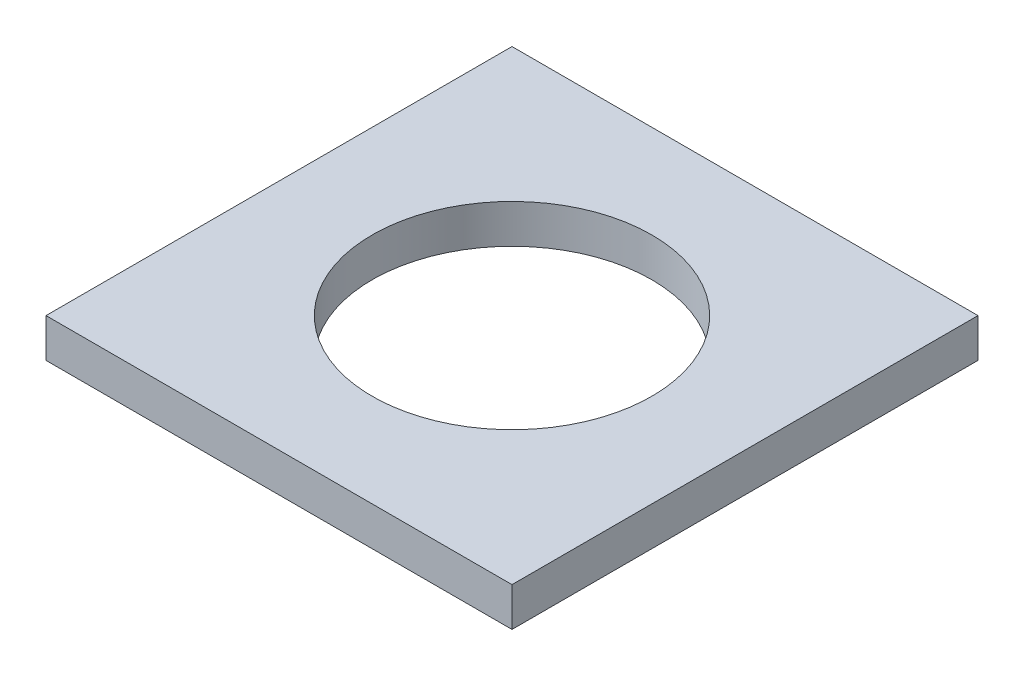
SolidWorks part; units mm, degrees
ref_plane "Front Plane" through (0, 0, 0) normal (0, 0, 1) x (1, 0, 0)
ref_plane "Top Plane" through (0, 0, 0) normal (0, 1, 0) x (1, 0, 0)
ref_plane "Right Plane" through (0, 0, 0) normal (1, 0, 0) x (0, 0, -1)
ref_plane "Plane1" through (0, 819.8956, 0) normal (0, 1, 0) x (1, 0, 0)
sketch "Sketch1" plane through (0, 819.8956, 0) normal (0, 1, 0) x (1, 0, 0)
  line L0 (581.2306, 380.693) -> (581.2306, 500.693)
  line L1 (581.2306, 500.693) -> (461.2306, 500.693)
  line L2 (461.2306, 500.693) -> (461.2306, 380.693)
  line L3 (461.2306, 380.693) -> (581.2306, 380.693)
  circle A0 centre (521.2306, 440.693) radius 36
  dimension "D1" = 72
  dimension "D2" = 60
  dimension "D3" = 120
  dimension "D4" = 60
  dimension "D5" = 120
extrude "Boss-Extrude1" add sketch "Sketch1" against normal blind 10
